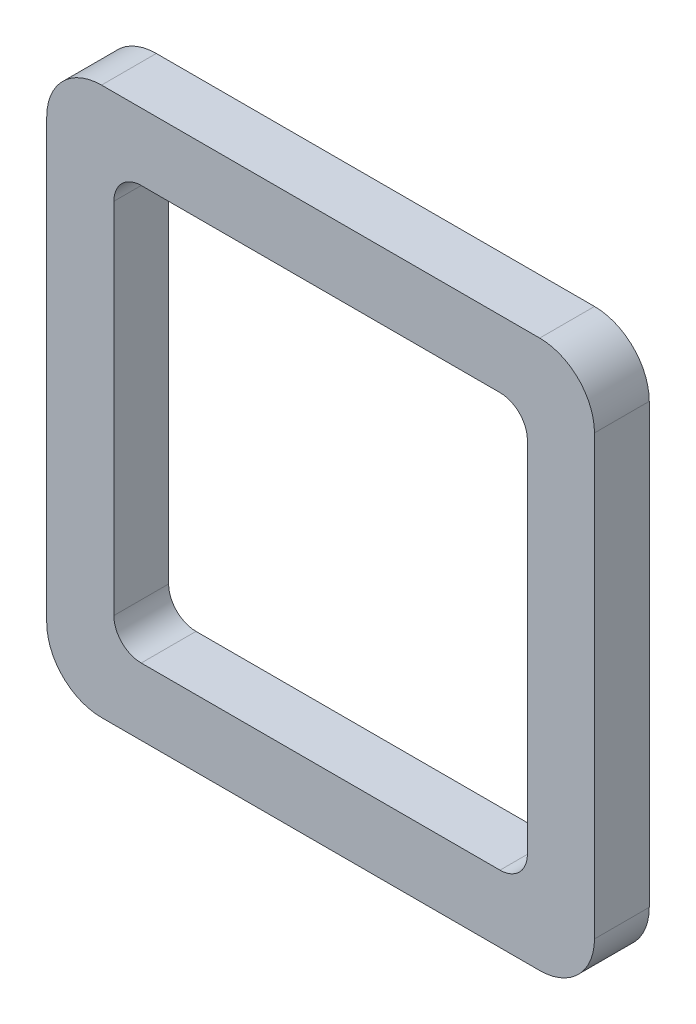
SolidWorks part; units mm, degrees
ref_plane "Front Plane" through (0, 0, 0) normal (0, 0, 1) x (1, 0, 0)
ref_plane "Top Plane" through (0, 0, 0) normal (0, 1, 0) x (1, 0, 0)
ref_plane "Right Plane" through (0, 0, 0) normal (1, 0, 0) x (0, 0, -1)
sketch "Sketch1" plane through (0, 0, 0) normal (0, 0, 1) x (1, 0, 0)
  line L1 (0, 0) -> (200, 0)
  line L2 (0, 0) -> (0, 200)
  line L3 (0, 200) -> (200, 200)
  line L4 (200, 0) -> (200, 200)
  line L5 (24.5, 175.5) -> (175.5, 175.5)
  line L6 (24.5, 175.5) -> (24.5, 24.5)
  line L7 (24.5, 24.5) -> (175.5, 24.5)
  line L8 (175.5, 175.5) -> (175.5, 24.5)
  dimension "D1" = 200
  dimension "D2" = 200
  dimension "D3" = 151
  dimension "D4" = 151
  dimension "D5" = 24.5
  dimension "D6" = 24.5
extrude "Boss-Extrude1" add sketch "Sketch1" along normal blind 20
fillet "Fillet1" radius 20 4 edges at (0, 0, 10) (200, 0, 10) (200, 200, 10) (0, 200, 10)
fillet "Fillet2" radius 10 4 edges at (175.5, 24.5, 10) (175.5, 175.5, 10) (24.5, 175.5, 10) (24.5, 24.5, 10)
